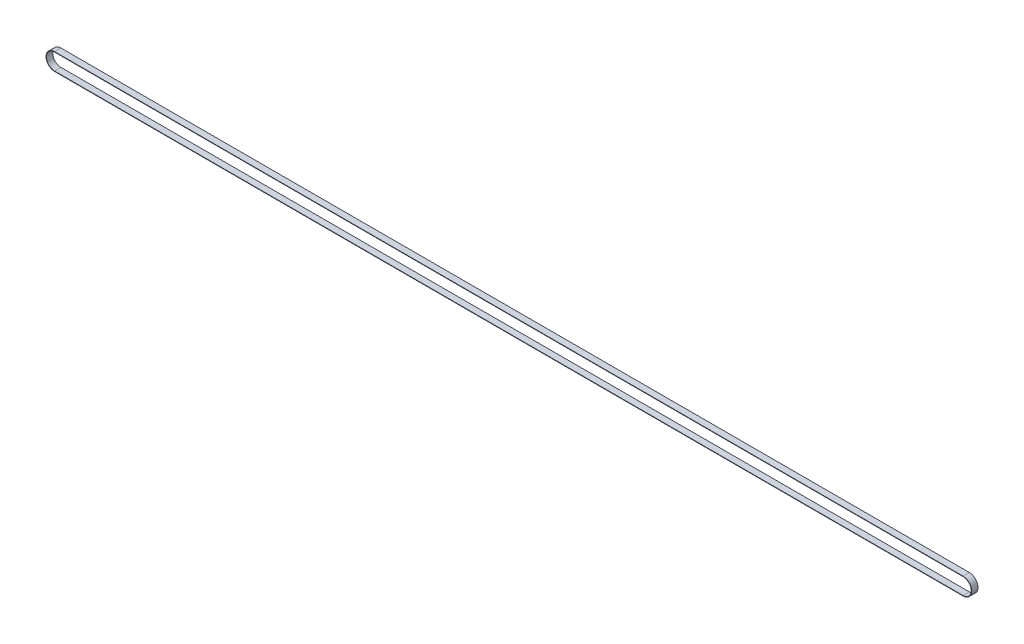
from build123d import *

# Parameters (mm, degrees)
EXTRUDE_1_DEPTH = 7.5


with BuildPart() as part:
    # 草图2 → 拉伸-薄壁1 (new, symmetric)
    with BuildSketch(Plane.XY):
        with BuildLine():
            Line((2155, -20.415), (0, -20.415))
            ThreePointArc((0, -20.415), (-20.415, 0), (0, 20.415))
            Line((0, 20.415), (2155, 20.415))
            ThreePointArc((2155, 20.415), (2175.415, 0), (2155, -20.415))
        make_face()
        with BuildLine():
            Line((2155, -19.415), (0, -19.415))
            ThreePointArc((0, -19.415), (-19.415, 0), (0, 19.415))
            Line((0, 19.415), (2155, 19.415))
            ThreePointArc((2155, 19.415), (2174.415, 0), (2155, -19.415))
        make_face(mode=Mode.SUBTRACT)
    extrude(amount=EXTRUDE_1_DEPTH, both=True)


solid = part.part
